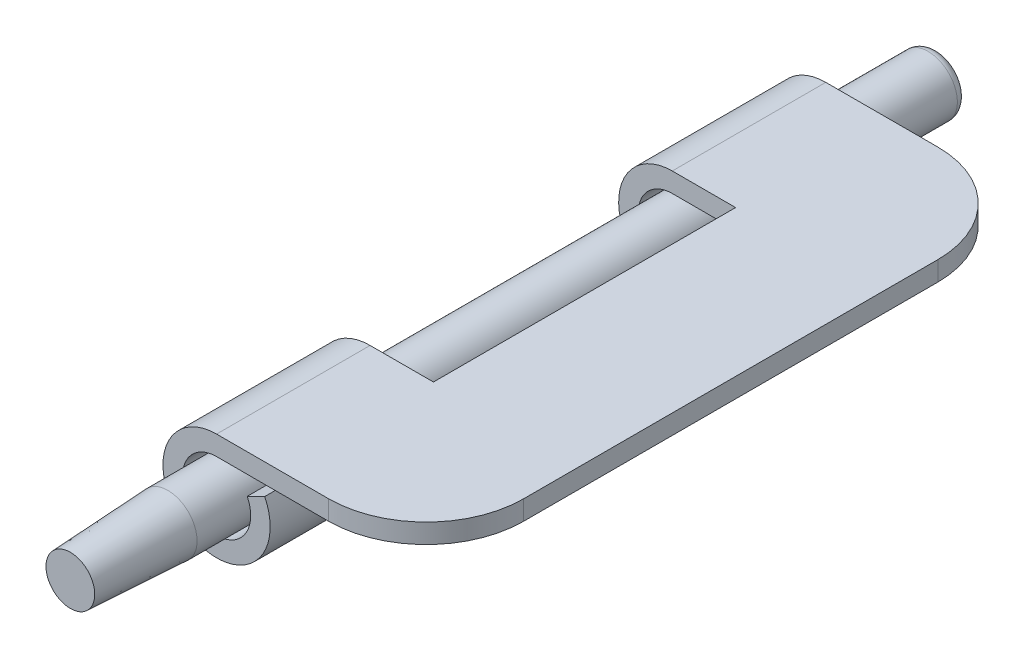
SolidWorks part; units mm, degrees
material "碳钢镀锌"
ref_plane "前视" through (0, 0, 0) normal (0, 0, 1) x (1, 0, 0)
ref_plane "上视" through (0, 0, 0) normal (0, 1, 0) x (1, 0, 0)
ref_plane "右视" through (0, 0, 0) normal (1, 0, 0) x (0, 0, -1)
sketch "草图3" plane through (0, 0, 0) normal (0, 0, 1) x (1, 0, 0)
  line L0 (21.5, 0) -> (0, 0)
  arc A0 (0, 0) -> (3.143, -1.96) centre (0, -3.5) ccw
  dimension "D2" = 7
  dimension "D1" = 21.5
extrude "拉伸-薄壁5" add sketch "草图3" along normal mid plane 62.5 thin contours L0 A0
sketch "草图4" plane through (0, 2, 0) normal (0, 1, 0) x (1, 0, 0)
  line L0 (-5.5, 31.25) -> (-5.5, -31.25) construction
  line L1 (-5.5, 15.5) -> (6.5, 15.5)
  line L2 (-5.5, 15.5) -> (-5.5, -15.5)
  line L3 (-5.5, -15.5) -> (6.5, -15.5)
  line L4 (6.5, 15.5) -> (6.5, -15.5)
  line L5 (21.5, 0) -> (-5.5, 0) construction
  line L6 (21.5, -31.25) -> (21.5, 31.25) construction
  dimension "D1" = 31
  dimension "D2" = 12
extrude "切除-拉伸1" cut sketch "草图4" against normal through all
ref_plane "基准面1" [suppressed] through (0, 0, 42.75) normal (0, 0, 1) x (1, 0, 0)
sketch "草图6" [suppressed] plane through (0, 0, 42.75) normal (0, 0, 1) x (1, 0, 0)
  circle A0 centre (0, -3.5) radius 3
  dimension "D1" = 6
extrude "凸台-拉伸3" [suppressed] add sketch "草图6" against normal blind 89 contours A0
chamfer "倒角1" [suppressed] distance 0.5 distance2 10
ref_plane "基准面2" through (0, 0, -42.75) normal (0, 0, -1) x (-1, 0, 0)
sketch "草图8" plane through (0, 0, -42.75) normal (0, 0, -1) x (-1, 0, 0)
  circle A0 centre (0, -3.5) radius 3
  dimension "D1" = 6
extrude "凸台-拉伸4" add sketch "草图8" against normal blind 89 separate body contours A0
chamfer "倒角2" distance 0.5 distance2 10 1 edges at (-3, -3.5, 46.25)
fillet "圆角1" radius 10 2 edges at (21.5, 1, -31.25) (21.5, 1, 31.25)
fillet "圆角2" radius 1 1 edges at (-3, -3.5, -42.75)
